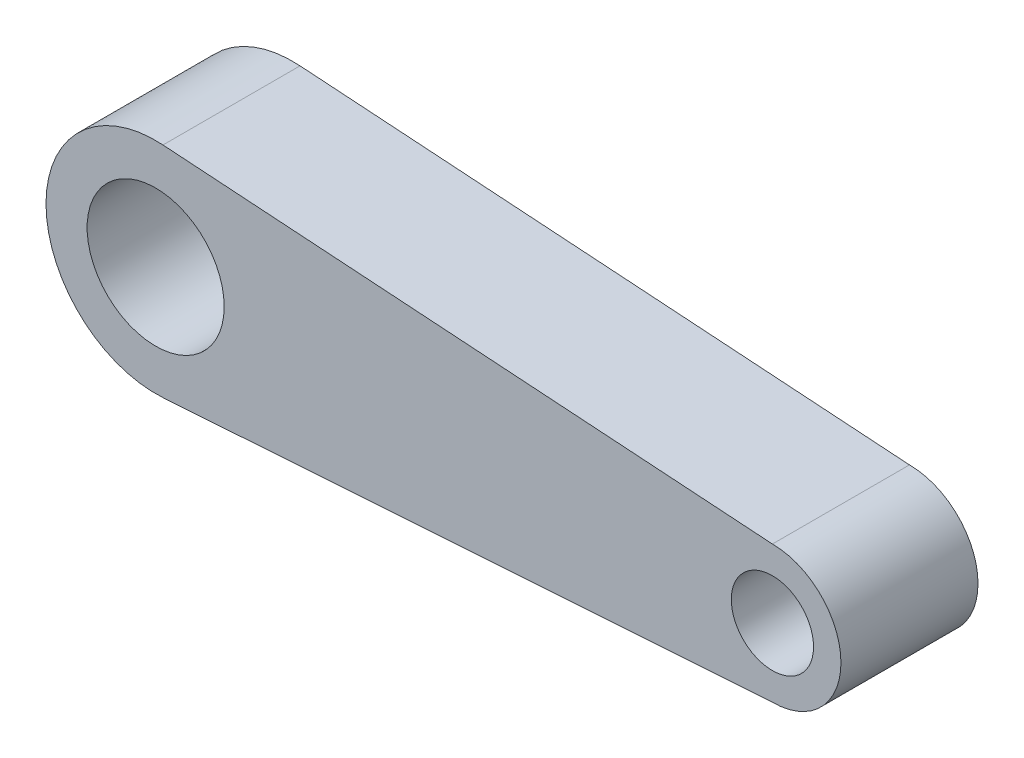
from build123d import *

# Parameters (mm, degrees)
SKETCH1_R           = 7.5
SKETCH1_R_2         = 4.5
BOSS_EXTRUDE1_DEPTH = 7.5


with BuildPart() as part:
    # Sketch1 → Boss-Extrude1 (new, symmetric)
    with BuildSketch(Plane.XY):
        with BuildLine():
            Line((0.80298849, 11.973103586), (67.5, 7.5))
            ThreePointArc((67.5, 7.5), (75, 0), (67.5, -7.5))
            Line((67.5, -7.5), (0.80298849, -11.973103586))
            ThreePointArc((0.80298849, -11.973103586), (-12, 0), (0.80298849, 11.973103586))
        make_face()
        Circle(SKETCH1_R, mode=Mode.SUBTRACT)
        with Locations((67.5, 0)):
            Circle(SKETCH1_R_2, mode=Mode.SUBTRACT)
    extrude(amount=BOSS_EXTRUDE1_DEPTH, both=True)


solid = part.part
